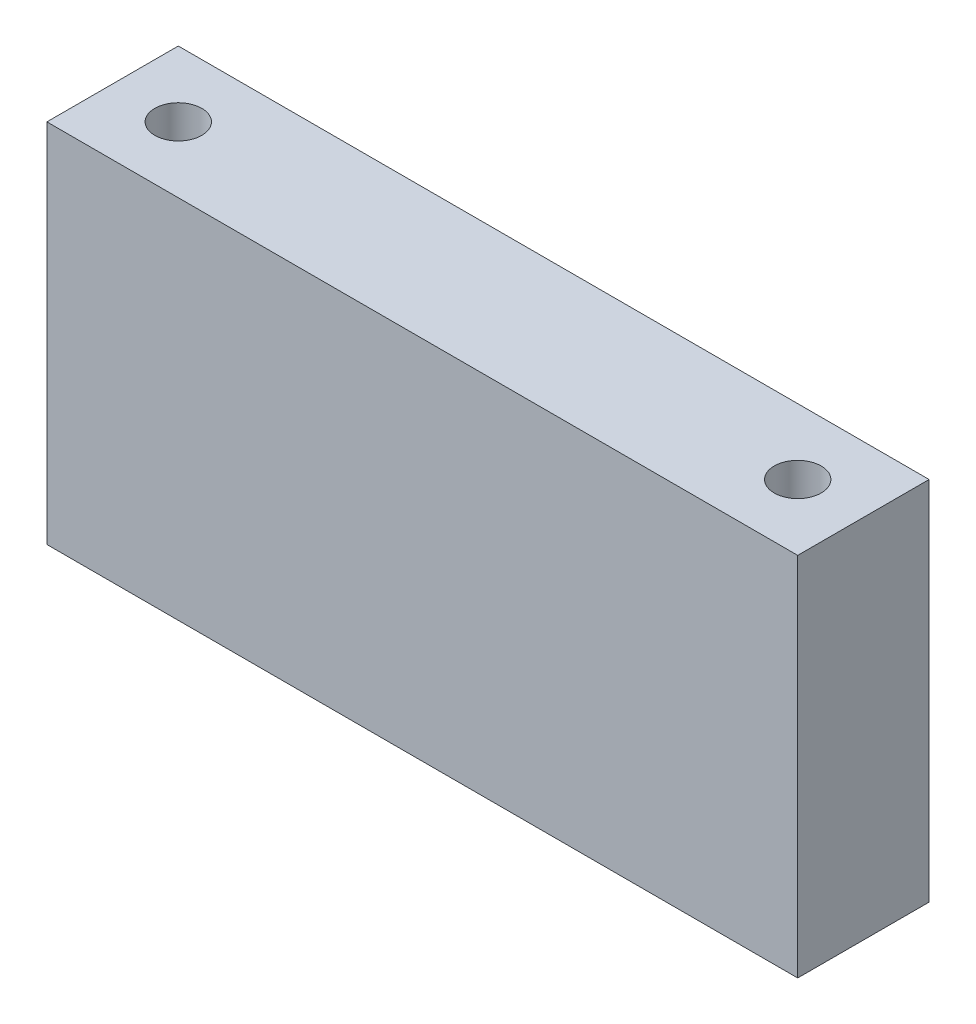
from build123d import *

# Parameters (mm, degrees)
SKETCH_1_W             = 80
SKETCH_1_H             = 39
EXTRUDE_1_DEPTH        = 14
HOLE_WIZARD_M6_1_D     = 5
HOLE_WIZARD_M6_1_DEPTH = 17
HOLE_WIZARD_M6_1_TIP   = 1.502151548
HOLE_WIZARD_M6_2_D     = 5
HOLE_WIZARD_M6_2_DEPTH = 17
HOLE_WIZARD_M6_2_TIP   = 1.502151548


with BuildPart() as part:
    # 草图1 → 凸台-拉伸1 (new body)
    with BuildSketch(Plane.XY):
        Rectangle(SKETCH_1_W, SKETCH_1_H)
    extrude(amount=EXTRUDE_1_DEPTH)

    # M6 螺纹孔1
    with Locations(Plane(origin=(0, -19.5, 0), x_dir=(-1, 0, 0), z_dir=(0, -1, 0))):
        with Locations((-21, -7), (21, -7)):
            Hole(HOLE_WIZARD_M6_1_D / 2, depth=HOLE_WIZARD_M6_1_DEPTH)
            with Locations((0, 0, -(HOLE_WIZARD_M6_1_DEPTH + HOLE_WIZARD_M6_1_TIP / 2))):  # 118° drill point
                Cone(0, HOLE_WIZARD_M6_1_D / 2, HOLE_WIZARD_M6_1_TIP, mode=Mode.SUBTRACT)

    # M6 螺纹孔2
    with Locations(Plane(origin=(0, 19.5, 0), x_dir=(1, 0, 0), z_dir=(0, 1, 0))):
        with Locations((-33, -7), (33, -7)):
            Hole(HOLE_WIZARD_M6_2_D / 2, depth=HOLE_WIZARD_M6_2_DEPTH)
            with Locations((0, 0, -(HOLE_WIZARD_M6_2_DEPTH + HOLE_WIZARD_M6_2_TIP / 2))):  # 118° drill point
                Cone(0, HOLE_WIZARD_M6_2_D / 2, HOLE_WIZARD_M6_2_TIP, mode=Mode.SUBTRACT)


solid = part.part
